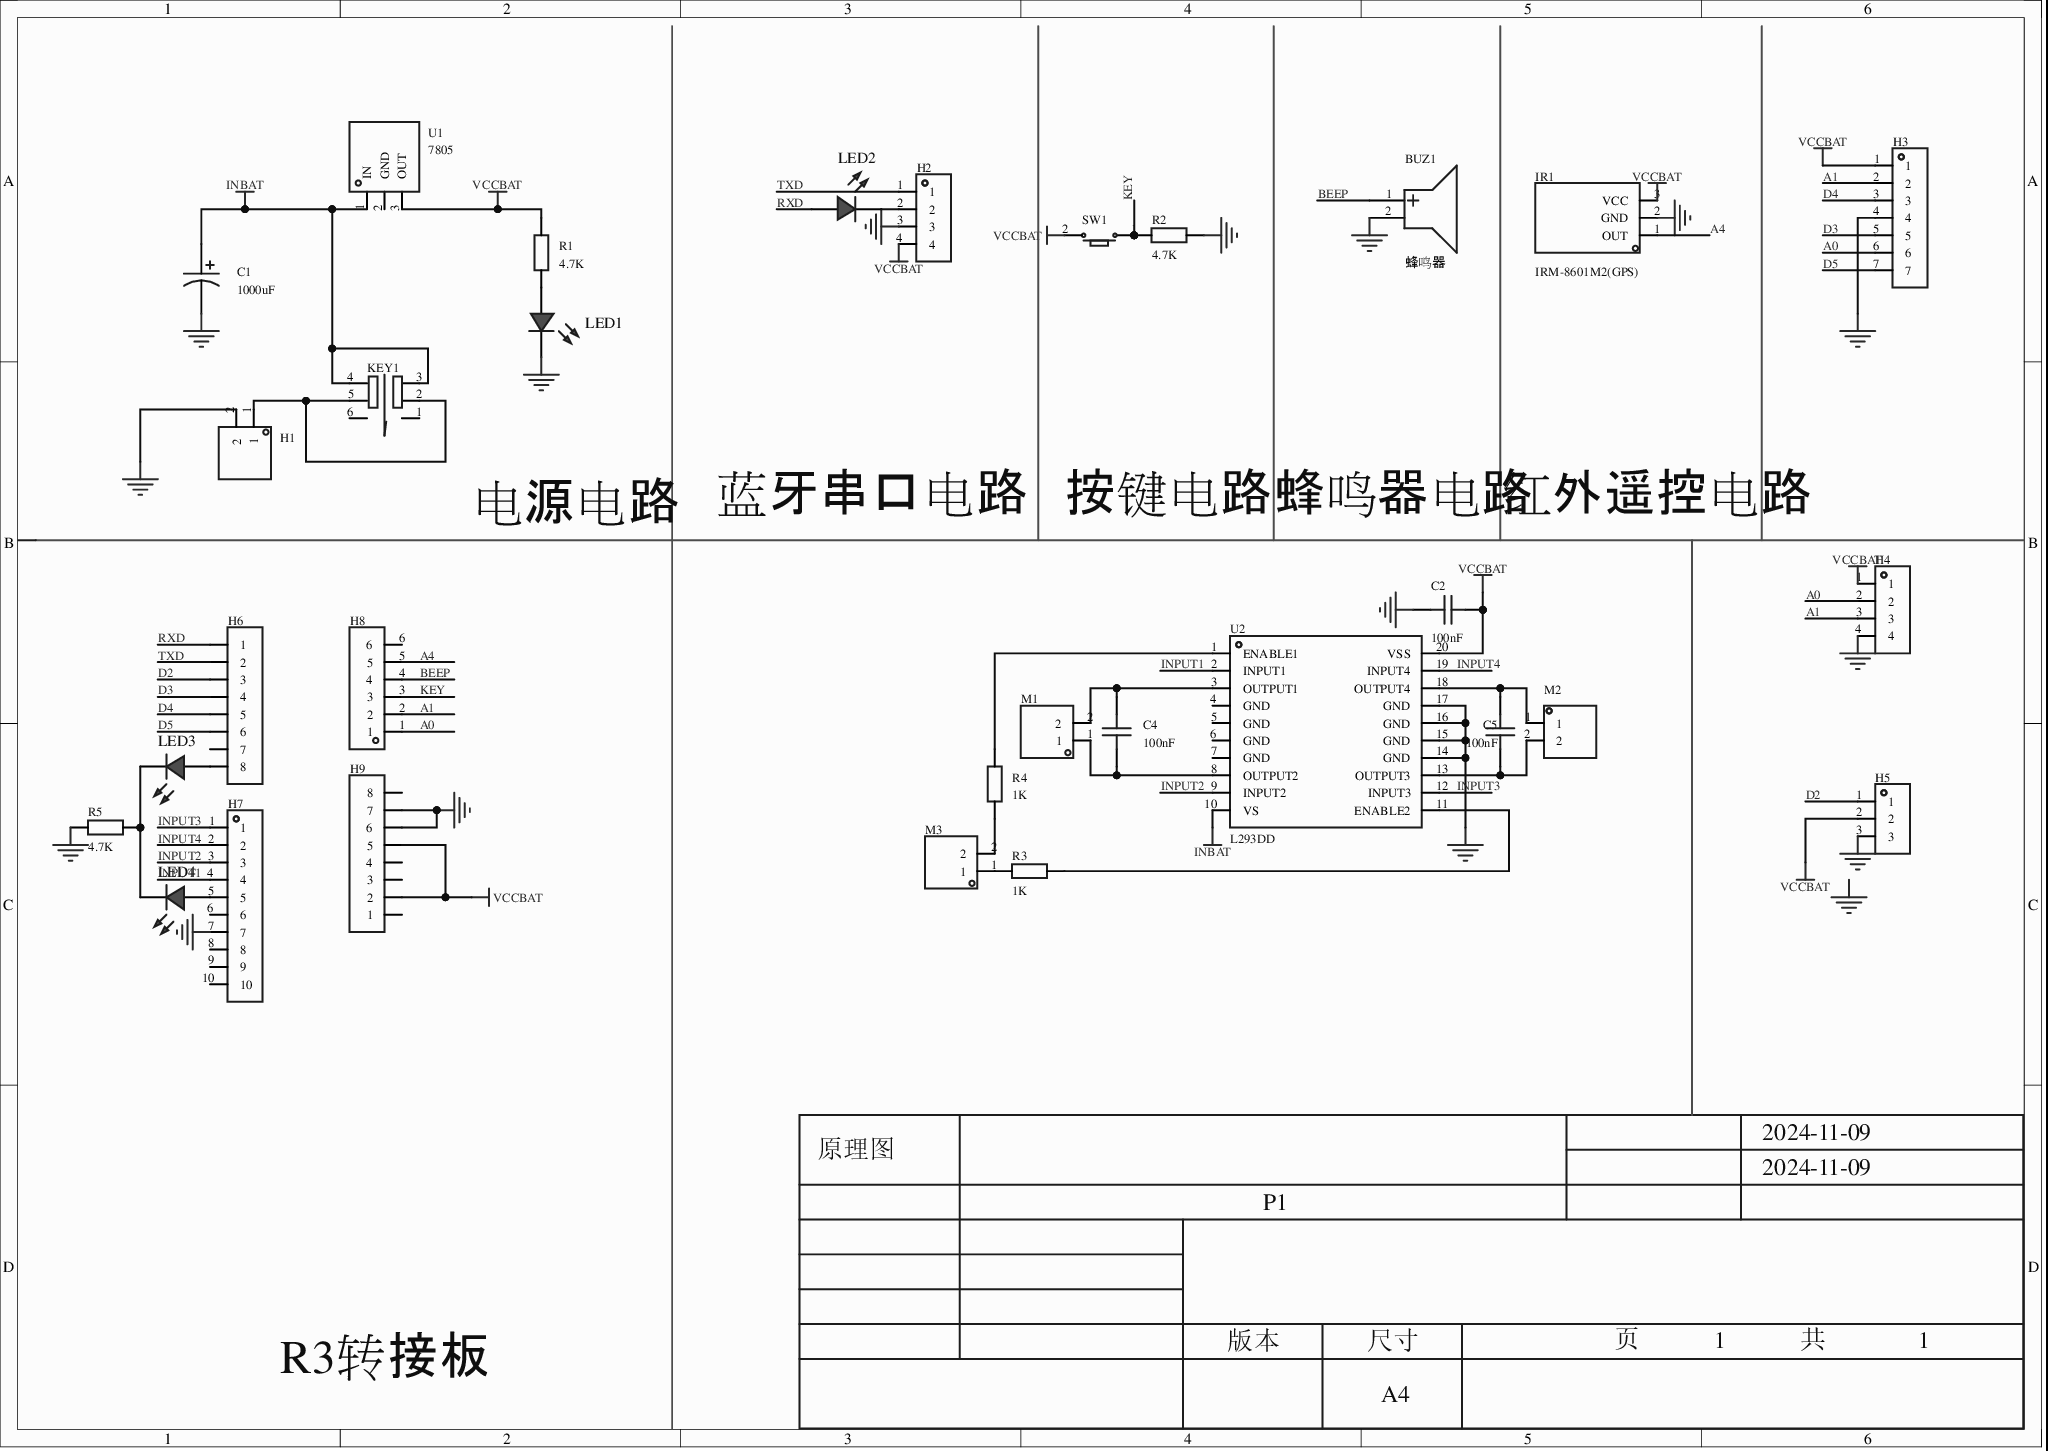
[diagram p0: MISC51932-3.schdoc]
# Altium project MISC51932-2.PrjPcb
1 sheet, 31 parts. Net scope: global (net labels, ports and power ports of the same name join across sheets).
Board file: MISC51932.pcbdoc

## Sheet MISC51932-3.schdoc
size 297 x 210 mm; Version: V1.0; @Project Name: MISC51932; @Page Count: 1; @Update Date: 2024-11-09; @Create Date: 2024-11-09; @Schematic Name: MISC51932; @Page No: 1; @Board Name: MISC51932; @Create Time: 14:43:30; @Update Time: 16:01:02

### Parts
BUZ1  蜂鸣器  [BUZ-TH_BD9.0-P5.00-D0.6-FD]
C1  1000uF  [CAP-TH_BD8.0-P3.50-D0.6-FD]
C2  100nF  [C0603]
C4  100nF  [C0603]
C5  100nF  [C0603]
H1  (no value)  [HDR-TH_2P-P2.54-V-M-1]
H2  (no value)  [HDR-TH_4P-P2.54-V-F]
H3  (no value)  [HDR-TH_7P-P2.54-V-M]
H4  (no value)  [HDR-TH_4P-P2.54-V-F]
H5  (no value)  [HDR-TH_3P-P2.54-V-F]
H6  (no value)  [HDR-TH_8P-P2.54-V-F-1]
H7  (no value)  [HDR-TH_10P-P2.54-V-F]
H8  (no value)  [HDR-TH_6P-P2.54-V-F]
H9  (no value)  [HDR-TH_8P-P2.54-V-F-1]
IR1  IRM-8601M2(GPS)  [SENSOR-TH_IRM-8601]
KEY1  自锁开关 5.8Z白灰白260G  [SW-TH_6P-L5.8-W5.8-P2.00-LS4.5-TR]  (value not drawn)
LED1  (no value)  [LED_0603]
LED2  (no value)  [LED_0603]
LED3  (no value)  [LED_0603]
LED4  (no value)  [LED_0603]
M1  (no value)  [HDR-TH_2P-P2.54-V-M-1]
M2  (no value)  [HDR-TH_2P-P2.54-V-M-1]
M3  (no value)  [HDR-TH_2P-P2.54-V-M-1]
R1  4.7K  [R0603]
R2  4.7K  [R0603]
R3  1K  [R0603]
R4  1K  [R0603]
R5  4.7K  [R0603]
SW1  (no value)  [Key_SMD_3x4x2]
U1  7805  [TO-220-3_L10.2-W4.5-P2.54-L-1]
U2  L293DD  [SOIC-20_L13.0-W7.6-P1.27-LS10.3-BL]

### Nets
GND: BUZ1.2(-) C1.2 C2.1 H1.2 H2.3 H3.4 H4.4 H5.3 H7.7 H9.6 H9.7 IR1.2(GND) LED1.1(C) R2.1 R5.2 U2.14(GND) U2.15(GND) U2.16(GND) U2.17(GND)
INBAT: C1.1 KEY1.3 KEY1.4 U1.1(IN) U2.10(VS)
VCCBAT: C2.2 H2.4 H3.1 H4.1 H5.2 H9.2 H9.5 IR1.3(VCC) R1.2 SW1.2 U1.3(OUT) U2.20(VSS)
A0: H3.6 H4.2 H8.1
A1: H3.2 H4.3 H8.2
A4: H8.5 IR1.1(OUT)
BEEP: BUZ1.1(+) H8.4
D2: H5.1 H6.3
D3: H3.5 H6.4
D4: H3.3 H6.5
D5: H3.7 H6.6
INPUT1: H7.4 U2.2(INPUT1)
INPUT2: H7.3 U2.9(INPUT2)
INPUT3: H7.1 U2.12(INPUT3)
INPUT4: H7.2 U2.19(INPUT4)
KEY: H8.3 R2.2 SW1.1
RXD: H6.1 LED2.2(A)
TXD: H2.1 H6.2
NetC4_1: C4.1 M1.1 U2.8(OUTPUT2)
NetC4_2: C4.2 M1.2 U2.3(OUTPUT1)
NetC5_1: C5.1 M2.1 U2.18(OUTPUT4)
NetC5_2: C5.2 M2.2 U2.13(OUTPUT3)
NetH1_1: H1.1 KEY1.2 KEY1.5
NetH2_2: H2.2 LED2.1(C)
NetH6_8: H6.8 LED3.2(A)
NetH7_5: H7.5 LED4.2(A)
NetLED1_2: LED1.2(A) R1.1
NetLED3_1: LED3.1(C) LED4.1(C) R5.1
NetM3_1: M3.1 R3.2
NetM3_2: M3.2 R4.2
NetR3_1: R3.1 U2.11(ENABLE2)
NetR4_1: R4.1 U2.1(ENABLE1)

Not connected (* = marked no-connect by the designer): H6 7; H7 6 8 9 10; H8 6; H9 1 3 4 8; KEY1 1 6; U1 2(GND); U2 4(GND) 5(GND) 6(GND) 7(GND)

### Notes on the sheet
- 电源电路
- 蓝牙串口电路
- 按键电路
- 蜂鸣器电路
- 红外遥控电路
- R3转接板
- Labels drawn without touching a wire or pin: GND
- 2024-11-09
- 原理图
- P1
- 版本
- 尺寸
- A4
- 页
- 1
- 共

### Library data of the parts
BUZ1 = 蜂鸣器: AddInBom: yes; ModelId: 13273335caac486e928bafb4d9fdf12d; ModelName: BUZ-TH_D9.0-H5.5-P5.0; ModelTransform: 354.33,354.33,0,90,0,0,-0.005,0,-177.165; Symbol: 蜂鸣器; Device: 蜂鸣器; LCSC Part Name: 蜂鸣器; SupplierPart: C9900020875; ManufacturerPart: 蜂鸣器; Supplier Footprint: 插件; JLCPCB Part Class: 扩展库; Supplier: LCSC; ConvertToPcb: yes; FootprintName: BUZ-TH_BD9.0-P5.00-D0.6-FD
C1 = SHW1000UF10V8X12: 容值:1000uF;精度:±20%;额定电压:10V;纹波电流:-;等效串联电阻:-;; Manufacturer: KNSCHA(科尼盛); AddInBom: yes; ModelId: a2c936ec27754f809f3966430e36f767; ModelName: CAP-TH_D8.0-H8.0-P3.50; ModelTransform: 314.96,314.862,0,180,0,0,0,0,-137.795; Tolerance: ±20%; Rated Voltage: 10V; φD: 8mm; L: 12mm; Lifetime @ Temp: 10000hrs@105℃; Symbol: SHW1000UF10V8X12; Device: SHW1000UF10V8X12; LCSC Part Name: 1000uF ±20% 10V; SupplierPart: C494548; ManufacturerPart: SHW1000UF10V8X12; Supplier Footprint: 插件,D8xL12mm; Datasheet: https://atta.szlcsc.com/upload/public/pdf/source/20200310/C494548_8AB2F4B606EB8D11D75E4665E4154421.pdf; Supplier: LCSC; ConvertToPcb: yes; FootprintName: CAP-TH_BD8.0-P3.50-D0.6-FD; Value: 1000uF; Ripple Current: -; Equivalent Series Resistance(ESR): -; Lead Spacing: 3.5mm
C2 C4 C5 = CAP_0603: ConvertToPcb: yes; SymbolName: CapAcitance; ModelId: ac125912035d415993ca9572d50418b1; ModelName: C0603_L1.6-W0.8-H0.8; ModelTransform: 62.992,31.496,0,0,0,0,0,0,0; Device: CAP_0603; AddInBom: yes; Supplier Footprint: 0603; FootprintName: C0603; Value: 100nF
H1 M1-M3 = HDR-M_2.54_1x2P: Symbol: 210S-1*2P L=11.6MMGold-plated black; ConvertToPcb: yes; ModelId: 79b2e9f2d70a4d68a1b7098f27c6d4c5; ModelName: HDR-M-2.54_1x2; ModelTransform: 200,100,0,0,0,0,0,0,-118.11; Device: HDR-M_2.54_1x2P; AddInBom: yes; SupplierPart: C124375; Supplier Footprint: 插件; FootprintName: HDR-TH_2P-P2.54-V-M-1
H2 H4 = HDR-F_2.54_1x4P: Symbol: 2.54-1*4P母; ConvertToPcb: yes; ModelId: d187812051054f85879fcaa51a310d8e; ModelTransform: 419.6842,98.464,0,0,0,0,0,0,-118.11; Device: HDR-F_2.54_1x4P; AddInBom: yes; SupplierPart: C2718488; Supplier Footprint: 插件; FootprintName: HDR-TH_4P-P2.54-V-F; ModelName: HDR-TH_4P-P2.54-V-F
H3 = HDR-M_2.54_1x7P: Symbol: PZ254V-11-07P; ConvertToPcb: yes; ModelId: 3f496cdc752348c6a5e9157bbaceaf96; ModelName: HDR-TH_7P-P2.54-M-LI-1X7P; ModelTransform: 690.1561,98.425,0,0,0,0,0,0,-118.11; Device: HDR-M_2.54_1x7P; AddInBom: yes; SupplierPart: C492406; Supplier Footprint: 插件; FootprintName: HDR-TH_7P-P2.54-V-M
H5 = HDR-F_2.54_1x3P: Symbol: PM254V-11-03-H85; ConvertToPcb: yes; ModelId: f3b3cc5aae9641bf9e56fc160cef875b; ModelName: HDR2.54-F-LI-1X3P; ModelTransform: 299.9994,100,0,0,0,0,0,0,-118.11; Device: HDR-F_2.54_1x3P; AddInBom: yes; SupplierPart: C541850; Supplier Footprint: 插件; FootprintName: HDR-TH_3P-P2.54-V-F
H6 H9 = HDR-F_2.54_1x8P: Symbol: Header-Female-2.54_1x8; AddInBom: yes; ModelId: 0f7e4d9227ef4fa08d5469c22cc70cdb; ModelName: HDR-F-2.54_1x8; ModelTransform: 799.99844,100,0,0,0,0,0,0,-118.11; Device: HDR-F_2.54_1x8P; ConvertToPcb: yes; FootprintName: HDR-TH_8P-P2.54-V-F-1; SupplierPart: C27438; Supplier Footprint: 插件
H7 = HDR-F_2.54_1x10P: Symbol: X5511FV-10-C70D30-1000; AddInBom: yes; ModelId: 08a5ee31ec6747838a696d2ac093ffa4; ModelName: HDR-TH_10P-P2.54-F-LI-1X10P; ModelTransform: 1009.87987,100,0,0,0,0,0,0,-125.984; Device: HDR-F_2.54_1x10P; ConvertToPcb: yes; FootprintName: HDR-TH_10P-P2.54-V-F; SupplierPart: C2684744; Supplier Footprint: 插件
H8 = HDR-F_2.54_1x6P: Symbol: Header-Female-2.54_1x6; ConvertToPcb: yes; ModelId: 0f5bcf94dcda47d085f24cdca1696fe9; ModelTransform: 619.684,94.488,0,0,0,0,0,0,-125.984; Device: HDR-F_2.54_1x6P; AddInBom: yes; SupplierPart: C40877; Supplier Footprint: 插件; FootprintName: HDR-TH_6P-P2.54-V-F; ModelName: HDR-TH_6P-P2.54-V-F
IR1 = IRM-8601M2(GPS): Manufacturer: EVERLIGHT(亿光); AddInBom: yes; ModelId: a53bc23b94404780ab3ec97d9b72604c; ModelTransform: 267.716,214.5665,0,0,0,0,0,-51.181,-157.48; Symbol: IRM-8601M2(GPS); Device: IRM-8601M2(GPS); LCSC Part Name: 红外线接收头 38KHz 直插; SupplierPart: C131222; ManufacturerPart: IRM-8601M2(GPS); Supplier Footprint: SIP-3-2.54mm; JLCPCB Part Class: 扩展库; Datasheet: https://atta.szlcsc.com/upload/public/pdf/source/20170918/C131222_1505726872476976233.pdf; Supplier: LCSC; ConvertToPcb: yes; FootprintName: SENSOR-TH_IRM-8601; ModelName: SENSOR-TH_IRM-8601
KEY1 = 自锁开关 5.8Z白灰白260G: 耐温260度; Symbol: Self-locking switch 5.8ZWhite and white260G; AddInBom: yes; ModelId: cd839ddf8c8d4e01911ba601e759d3e9; ModelTransform: 228.346,228.346,0,0,0,0,0,0,-137.795; Device: 自锁开关 5.8Z白灰白260G; LCSC Part Name: 自锁开关 5.8Z白灰白 260G  5.8*5.8mm; SupplierPart: C56857; ManufacturerPart: 自锁开关 5.8Z白灰白260G; Supplier Footprint: 插件; Supplier: LCSC; ConvertToPcb: yes; FootprintName: SW-TH_6P-L5.8-W5.8-P2.00-LS4.5-TR; ModelName: SW-TH_6P-L5.8-W5.8-P2.00-LS4.5-TR
LED1-LED4 = LED_0603-R: Symbol: LED_R; Convert to PCB: yes; 3D Model: dd8257b0d61a4cd7b68939a056e08095; 3D Model Transform: 58.72,29.4,22.03,0,0,0,0,0,0; ModelName: LED-0603_R; Device: LED_0603-R; Add into BOM: yes; Supplier Footprint: 0603; FootprintName: LED_0603
R1-R5 = Res_0603: Symbol: 电阻; ConvertToPcb: yes; ModelId: fc143cca1e79419f9cd78b61e9279f08; ModelTransform: 31.8897,63.7794,0,90,0,0,0,0,0; Device: Res_0603; AddInBom: yes; Supplier Footprint: 0603; FootprintName: R0603; ModelName: R0603
  R1 R2 R5: Value: 4.7K
  R3 R4: Value: 1K
SW1 = Key_SMD_3x4x2: ConvertToPcb: yes; SymbolName: 轻触按键x2; ModelId: 63599cce708d48afbce1b0db003544770819f05c4eef4c71ace90d822a990e87; ModelName: SW-SMD_L4.0-W2.9-H2-LS5.0; ModelTransform: 196.85,114.17,79.13,0,0,0,0,0,0; Device: Key_SMD_3x4x2; AddInBom: yes; Supplier Footprint: SMD; FootprintName: Key_SMD_3x4x2
U1 = 7805: 输出类型:固定;最大输入电压:35V;输出电压:5V;最大输出电流:1.5A;电源纹波抑制比(PSRR):62dB@(120Hz);输出极性:正极;; Manufacturer: SY(顺烨); Symbol: 7805_C4944936; AddInBom: yes; ModelId: 0369bc25c9bd44718af72a1d71ffd3cd; ModelTransform: 401.574,177.204,0,0,0,0,0,24.606,-196.85; Output Type: 固定; Maximum Input Voltage: 35V; Output Voltage: 5V; MAX Output Current: 1.5A; Output Polarity: 正极; Device: 7805; LCSC Part Name: 输入35V 输出5V 1.5A; SupplierPart: C4944936; ManufacturerPart: 7805; Supplier Footprint: TO-220AB; JLCPCB Part Class: 扩展库; Datasheet: https://atta.szlcsc.com/upload/public/pdf/source/20220719/323A3F14557C229271C454C7C0F759A5.pdf; Supplier: LCSC; ConvertToPcb: yes; FootprintName: TO-220-3_L10.2-W4.5-P2.54-L-1; ModelName: TO-220-3_L10.2-W4.5-P2.54-L-1; Power Supply Rejection Ratio (PSRR): 62dB@(120Hz); Dropout Voltage: -; standby current: -; Noise: -; Feature: -; Operating Temperature: -; Number of Outputs: -
U2 = L293DD_C2971293: 具有二极管的推挽四通道驱动器; Manufacturer: ST(意法半导体); AddInBom: yes; ModelId: fc022553ecdc4755a737d639ae95109c; ModelName: SOIC-20_L12.8-W7.5-H2.7-LS10.3-P1.27; ModelTransform: 503.936,409.68154,0,0,0,0,0,0,0; Symbol: L293DD_C2971293; Device: L293DD_C2971293; LCSC Part Name: L293DD; SupplierPart: C2971293; ManufacturerPart: L293DD; Supplier Footprint: SOIC-20-300mil; JLCPCB Part Class: 扩展库; Datasheet: https://atta.szlcsc.com/upload/public/pdf/source/20140724/1457707157802.pdf; Supplier: LCSC; ConvertToPcb: yes; FootprintName: SOIC-20_L13.0-W7.6-P1.27-LS10.3-BL